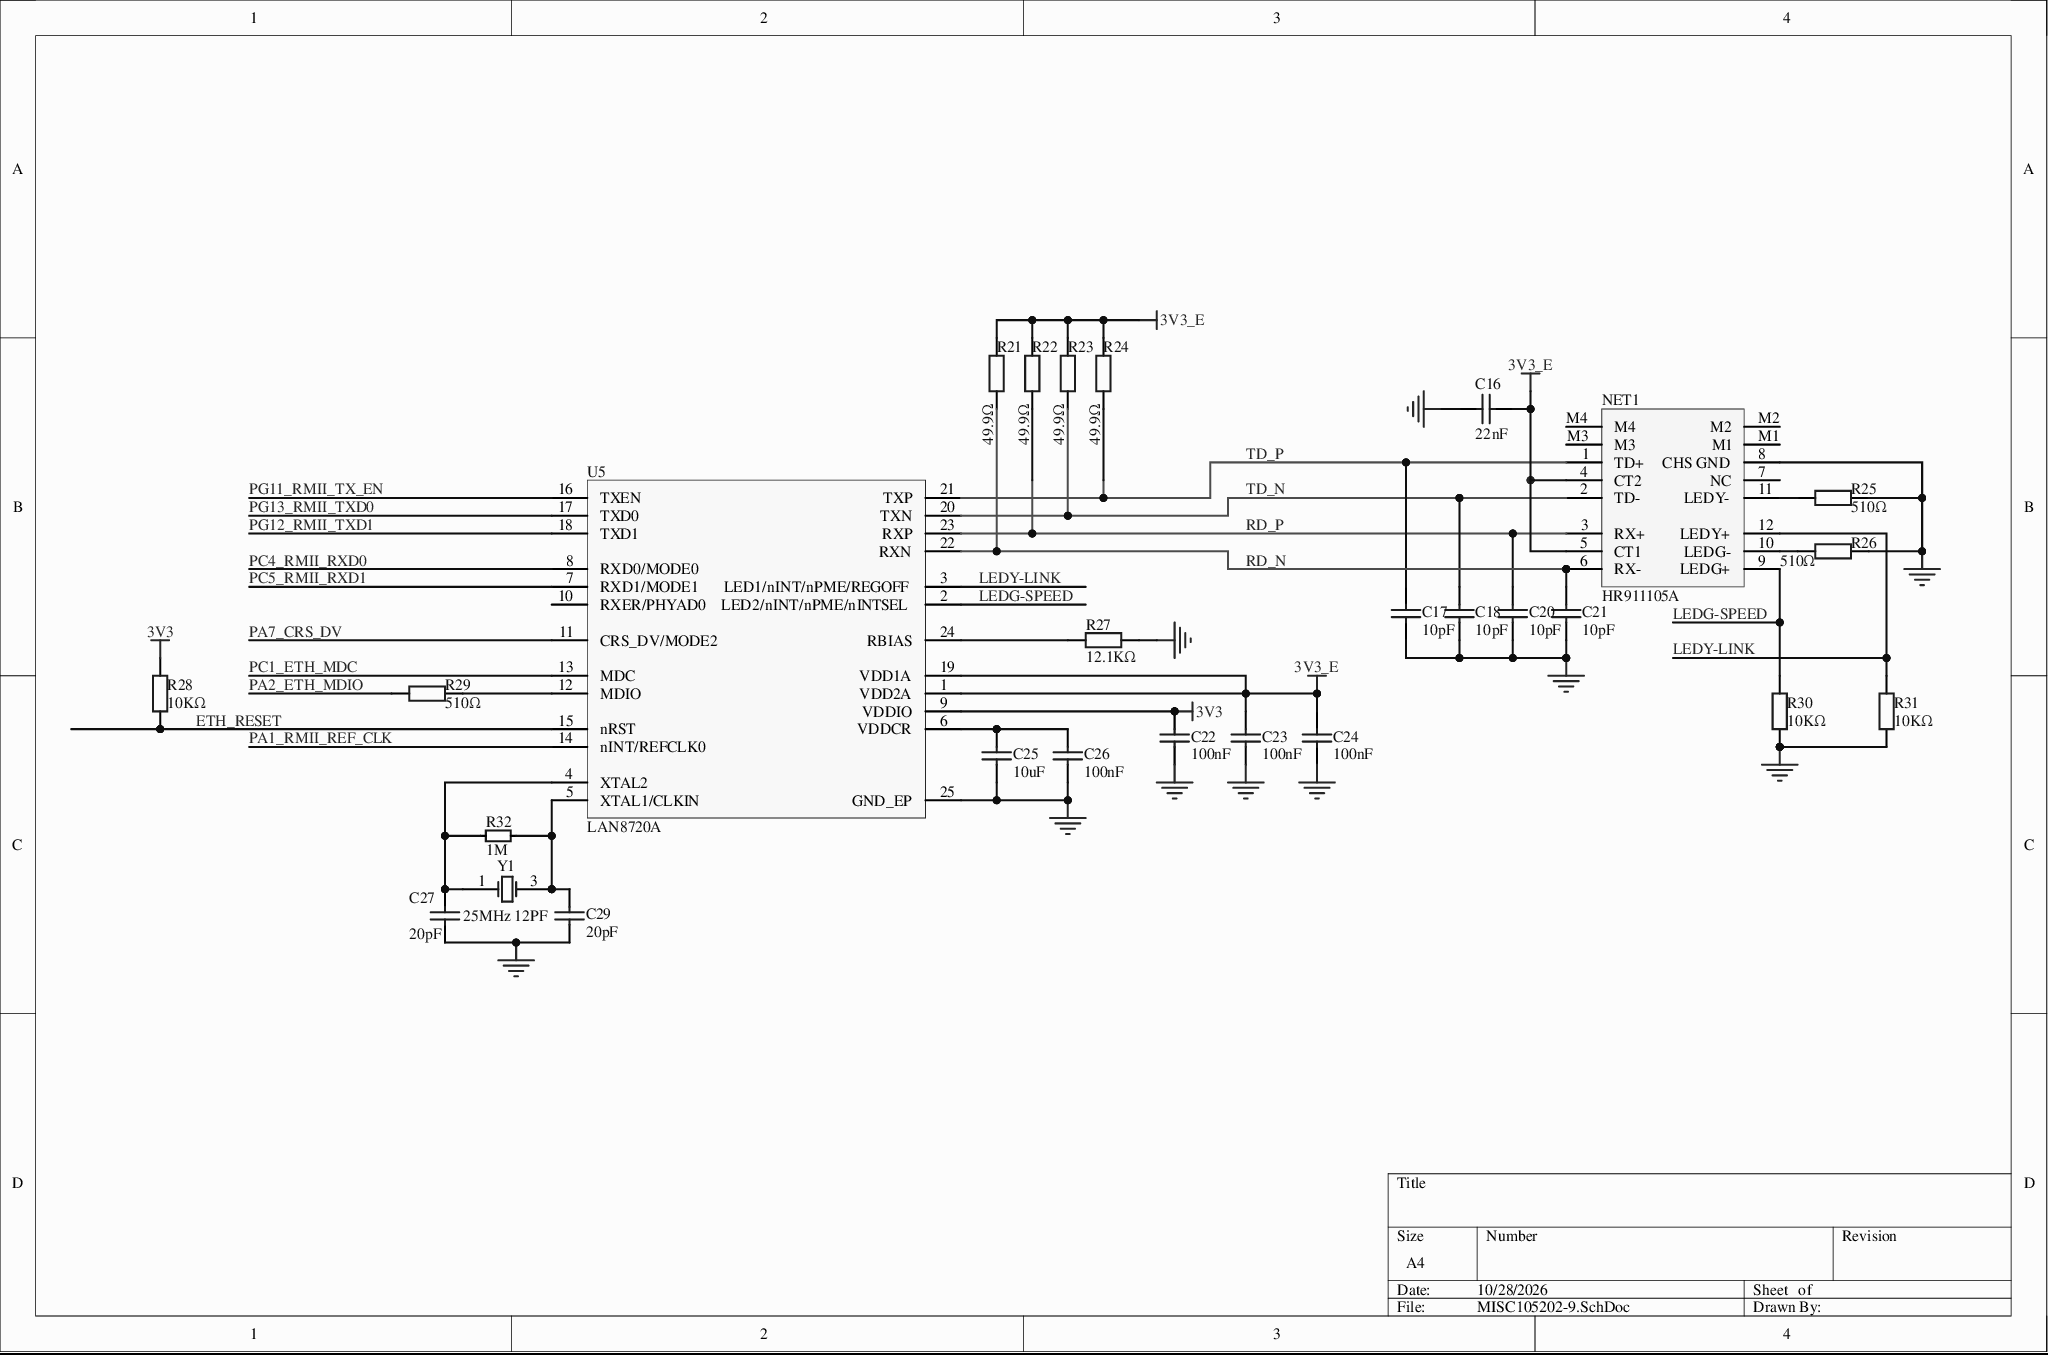
[diagram p0: MISC105202-9.SchDoc]
# Altium project MISC105202-19.PrjPCB (part 2 of 3)

## Sheet MISC105202-9.SchDoc
size A4

### Parts
C16  22nF  [0603_C]
C17  10pF  [0603_C]
C18  10pF  [0603_C]
C20  10pF  [0603_C]
C21  10pF  [0603_C]
C22  100nF  [0603_C]
C23  100nF  [0603_C]
C24  100nF  [0603_C]
C25  10uF  [0603_C]
C26  100nF  [0603_C]
C27  20pF  [0402_C]
C29  20pF  [0402_C]
NET1  HR911105A  [RJ45]
R21  49.9Ω  [0603_R]
R22  49.9Ω  [0603_R]
R23  49.9Ω  [0603_R]
R24  49.9Ω  [0603_R]
R25  510Ω  [0603_R]
R26  510Ω  [0603_R]
R27  12.1KΩ  [0603_R]
R28  10KΩ  [0603_R]
R29  510Ω  [0603_R]
R30  10KΩ  [0603_R]
R31  10KΩ  [0603_R]
R32  1M  [0402_R]
U5  LAN8720A  [QFN-24_4X4x05P]
Y1  25MHz 12PF  [SMD-3225_4P]

### Nets
3V3: C22.2 R28.1 U5.9(VDDIO)
3V3_E: C16.1 C23.2 C24.2 NET1.4(CT2) NET1.5(CT1) R21.2 R22.2 R23.2 R24.2 U5.1(VDD2A) U5.19(VDD1A)
GND: C16.2 C17.2 C18.2 C20.2 C21.2 C22.1 C23.1 C24.1 C25.1 C26.1 C27.2 C29.2 NET1.8(CHS_GND) R25.2 R26.2 R27.2 R30.2 R31.1 U5.25(GND_EP)
ETH_RESET: R28.2 U5.15(nRST)
LEDG-SPEED: NET1.9(LEDG+) R30.1 U5.2(LED2/nINT/nPME/nINTSEL)
LEDY-LINK: NET1.12(LEDY+) R31.2 U5.3(LED1/nINT/nPME/REGOFF)
PA1_RMII_REF_CLK: U5.14(nINT/REFCLK0)
PA2_ETH_MDIO: R29.1
PA7_CRS_DV: U5.11(CRS_DV/MODE2)
PC1_ETH_MDC: U5.13(MDC)
PC4_RMII_RXD0: U5.8(RXD0/MODE0)
PC5_RMII_RXD1: U5.7(RXD1/MODE1)
PG11_RMII_TX_EN: U5.16(TXEN)
PG12_RMII_TXD1: U5.18(TXD1)
PG13_RMII_TXD0: U5.17(TXD0)
RD_N: C21.1 NET1.6(RX-) R21.1 U5.22(RXN)
RD_P: C20.1 NET1.3(RX+) R22.1 U5.23(RXP)
TD_N: C18.1 NET1.2(TD-) R23.1 U5.20(TXN)
TD_P: C17.1 NET1.1(TD+) R24.1 U5.21(TXP)
NetC25_2: C25.2 C26.2 U5.6(VDDCR)
NetC27_1: C27.1 R32.2 U5.4(XTAL2) Y1.1(OSC1)
NetC29_1: C29.1 R32.1 U5.5(XTAL1/CLKIN) Y1.3(OSC2)
NetNET1_10: NET1.10(LEDG-) R26.1
NetNET1_11: NET1.11(LEDY-) R25.1
NetR27_1: R27.1 U5.24(RBIAS)
NetR29_2: R29.2 U5.12(MDIO)

Not connected (* = marked no-connect by the designer): NET1 7(NC) M1 M2 M3 M4; U5 10(RXER/PHYAD0)

### Layout directives
differential pair: RD_N, RD_P, TD_N, TD_P
rule Matched Net Lengths [Tolerance = 100mil]: RD_N, RD_P, TD_N, TD_P

### Library data of the parts
C16 = 0603 22nF (223) 10% 50V: 贴片电容; ComponentLink1Description: supplier link; Package: 0603; Supplier: LC; SuppliersPartNumber: C21122
C17 C18 C20 C21 = 0603 10pF (100) 5% 50V: 贴片电容; ComponentLink1Description: supplier link; Package: 0603; Supplier: LC; SuppliersPartNumber: C1634
C22-C24 C26 = 0603 100nF (104) 10% 50V: 贴片电容; ComponentLink1Description: supplier link; Package: 0603; Supplier: LC; SuppliersPartNumber: C14663
C25 = 0603 10uF (106) 10% 10V: 贴片电容; ComponentLink1Description: supplier link; Package: 0603; Supplier: LC; SuppliersPartNumber: C19702
C27 C29 = Cap Semi: Capacitor (Semiconductor SIM Model); Published: 8-Jun-2000; LatestRevisionDate: 29-May-2009; LatestRevisionNote: IPC-7351 Footprint Added.; PackageReference: C1206; PackageDescription: Chip Capacitor; Publisher: Altium Limited
R21-R24 = 0603 49.9Ω (49R9) 1%: 贴片电阻; ComponentLink1Description: supplier link; Package: 0603; Supplier: LC; SuppliersPartNumber: C23185
R25 R26 R29 = 0603 510Ω (5100) 1%: 贴片电阻; ComponentLink1Description: supplier link; Package: 0603; Supplier: LC; SuppliersPartNumber: C23193
R27 = 0603 12KΩ (1202) 1%: 贴片电阻; ComponentLink1Description: supplier link; Package: 0603; Supplier: LC; SuppliersPartNumber: C22790
R28 R30 R31 = 0603 10KΩ (1002) 1%: 贴片电阻; ComponentLink1Description: supplier link; Package: 0603; Supplier: LC; SuppliersPartNumber: C25804
R32 = Reszte: Resistor
U5 = LAN8742A-CZ-TR: LAN8742A-CZ-TR - Small Footprint RMII 10/100 Ethernet, Transceiver with HP Auto-MDIX and flexPWR Technology SQFN-24; Manuf_1: MICROCHIP; Order: LAN8742A-CZ-TR; Manuf_Part_1: LAN8742A-CZ-TR; Distrib: MICROCHIP
Y1 = SMD-3225_4P  25MHZ 12PF 10PPM: 贴片晶振; ComponentLink1Description: supplier link; Package: SMD-3225_4P; Supplier: LC; SuppliersPartNumber: C9006

## Sheet MISC105202-21.SchDoc
size B
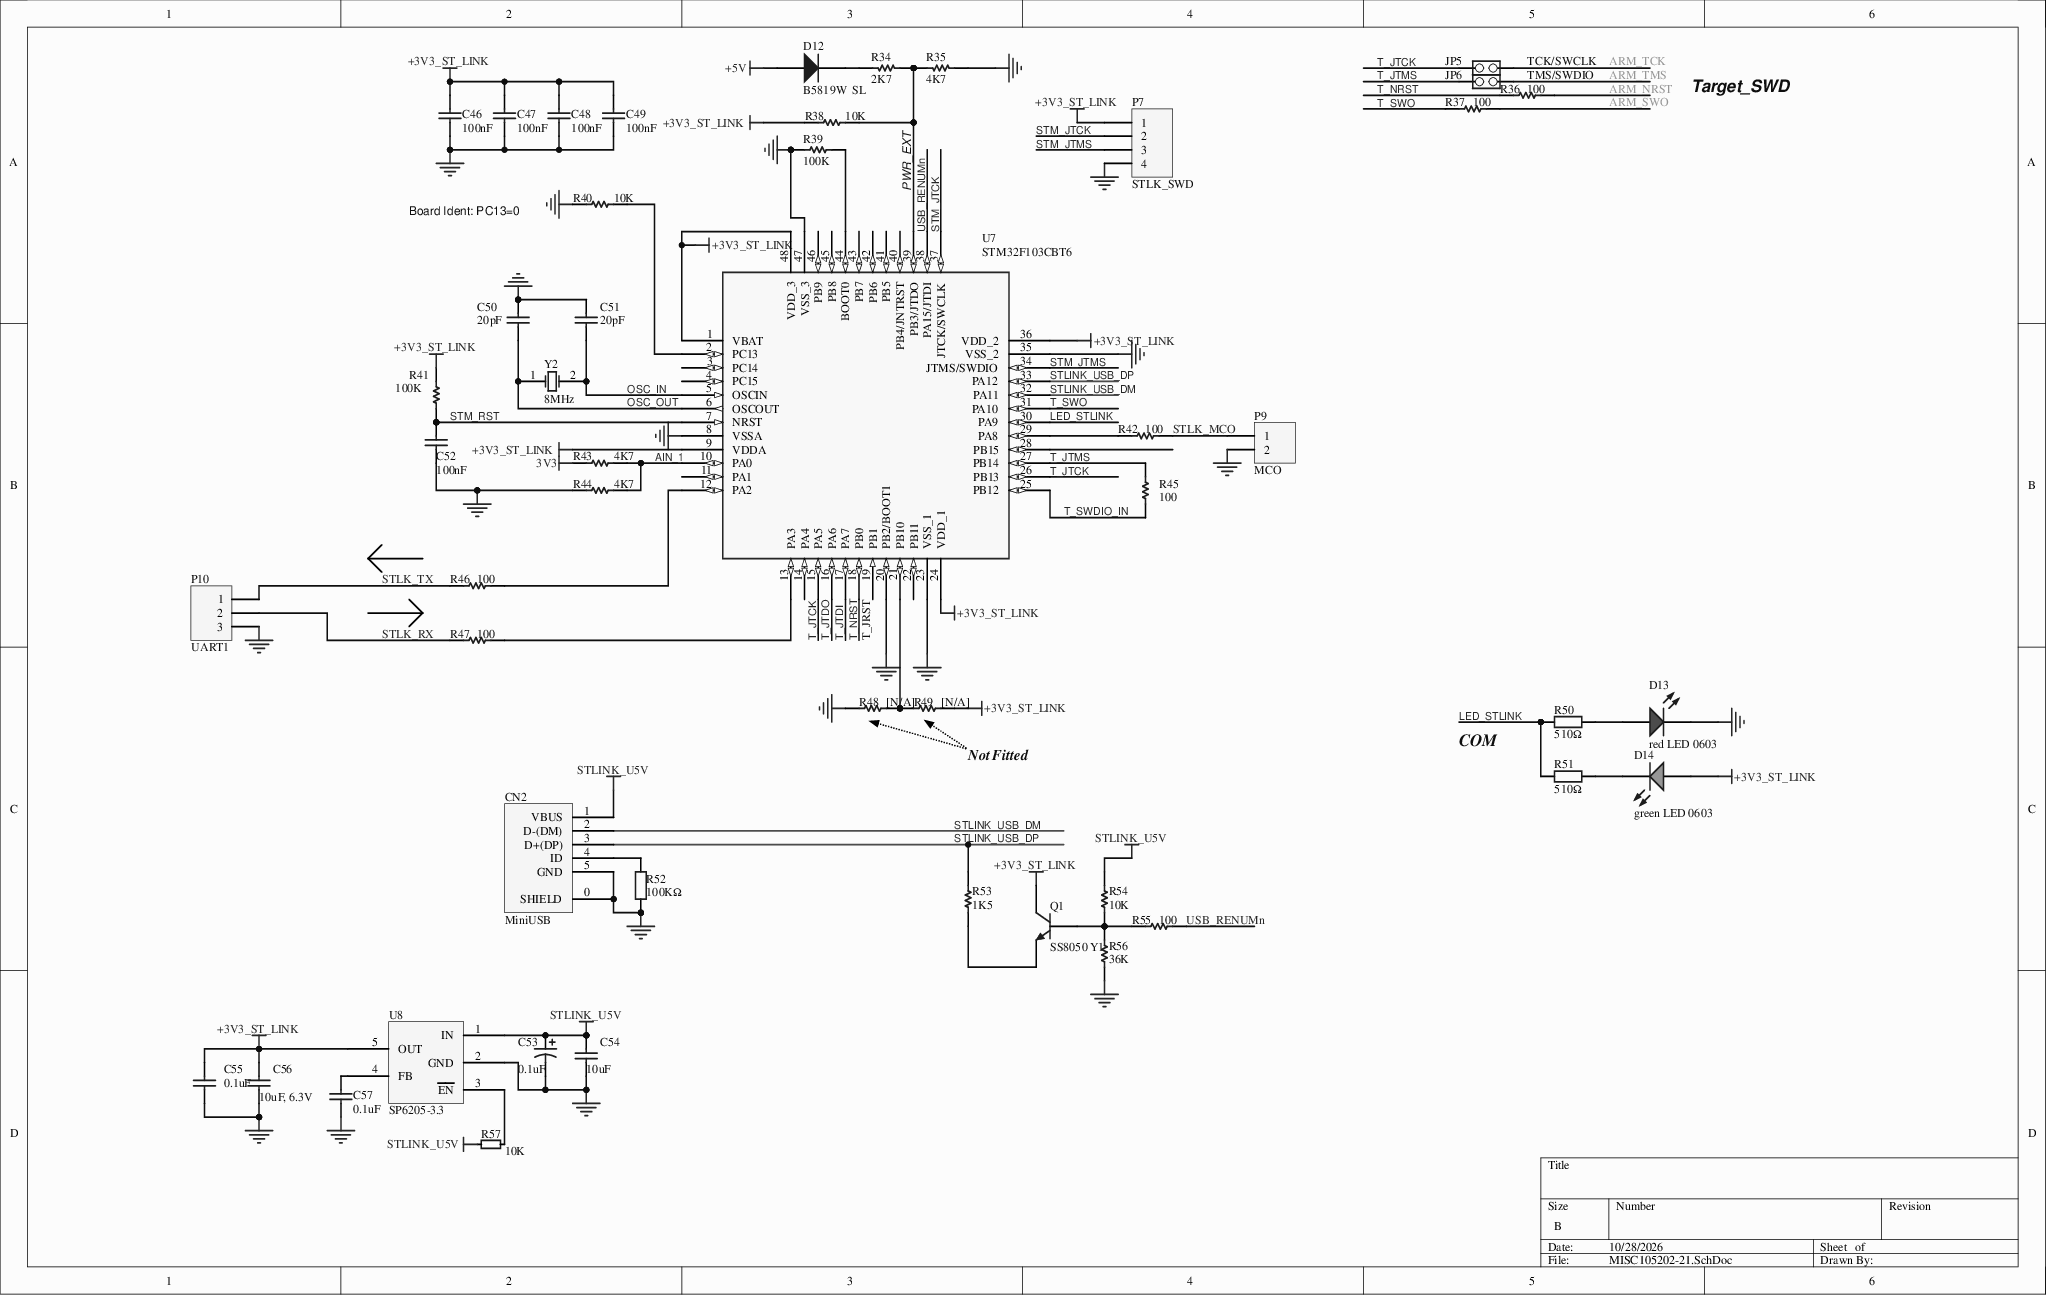
[diagram p1: MISC105202-21.SchDoc]

### Parts
C46  100nF  [0603_C]
C47  100nF  [0603_C]
C48  100nF  [0603_C]
C49  100nF  [0603_C]
C50  20pF  [0603_C]
C51  20pF  [0603_C]
C52  100nF  [0603_C]
C53  0.1uF  [0402_C]
C54  10uF  [0402_C]
C55  value 0.1uF  [0603_C]  (hidden comment: 0.1uF,25V)
C56  10uF, 6.3V  [0402_C]
C57  0.1uF  [0402_C]
CN2  MiniUSB  [Mini-USB-AB]
D12  B5819W  SL  [SOD-123]
D13  red LED 0603  [0603_LED_S1]
D14  green LED 0603  [0603_LED_S1]
JP5  (no value)  [HDR1X2]
JP6  (no value)  [HDR1X2]
P7  STLK_SWD  [127*4]
P9  MCO  [HDR1X2]
P10  UART1  [HDR1X3]
Q1  SS8050 Y1  [SOT-23(SOT-23-3)]
R34  2K7  [0603_R]
R35  4K7  [0603_R]
R36  100  [0603_R]
R37  100  [0603_R]
R38  10K  [0603_R]
R39  100K  [0603_R]
R40  10K  [0603_R]
R41  100K  [0603_R]
R42  100  [0603_R]
R43  4K7  [0603_R]
R44  4K7  [0603_R]
R45  100  [0603_R]
R46  100  [0603_R]
R47  100  [0603_R]
R48  [N/A]  [0603_R]
R49  [N/A]  [0603_R]
R50  510Ω  [0603_R]
R51  510Ω  [0603_R]
R52  100KΩ  [0603_R]
R53  1K5  [0603_R]
R54  10K  [0603_R]
R55  100  [0603_R]
R56  36K  [0603_R]
R57  10K  [0402_R]
U7  STM32F103CBT6  [LQFP-48_7x7x05P]
U8  SP6205-3.3  [SOT23-5]
Y2  8MHz  [SMD-5032_2P]

### Nets
3V3: R43.1
+3V3_ST_LINK: C46.2 C47.2 C48.2 C49.2 C55.2 C56.2 D14.A P7.1 Q1.3(C) R38.1 R41.2 R49.1 U7.1(VBAT) U7.9(VDDA) U7.24(VDD_1) U7.36(VDD_2) U7.48(VDD_3) U8.5(OUT)
+5V: D12.1(A)
GND: C46.1 C47.1 C48.1 C49.1 C50.2 C51.2 C52.1 C53.2 C54.1 C55.1 C56.1 C57.1 CN2.0(SHIELD) CN2.5(GND) D13.K P7.4 P9.2 P10.3 R35.2 R39.1 R40.1 R44.1 R48.2 R52.1 R56.1 U7.8(VSSA) U7.20(PB2/BOOT1) U7.23(VSS_1) U7.35(VSS_2) U7.47(VSS_3) U8.2(GND)
STLINK_U5V: C53.1 C54.2 CN2.1(VBUS) R54.2 R57.2 U8.1(IN)
AIN_1: R43.2 R44.2 U7.10(PA0)
ARM_NRST: R36.2
ARM_SWO: R37.2
ARM_TCK: JP5.2(NO)
ARM_TMS: JP6.2(NO)
LED_STLINK: R50.1 R51.1 U7.30(PA9)
OSC_IN: C51.1 U7.5(OSCIN) Y2.2(OSC2)
OSC_OUT: C50.1 U7.6(OSCOUT) Y2.1(OSC1)
STLINK_USB_DM: CN2.2(D-(DM)) U7.32(PA11)
STLINK_USB_DP: CN2.3(D+(DP)) R53.1 U7.33(PA12)
STLK_MCO: P9.1 R42.2
STLK_RX: P10.2 R47.1  [project net PA9_U1T]
STLK_TX: P10.1 R46.1  [project net PA10_U1R]
STM_JTCK: P7.2 U7.37(JTCK/SWCLK)
STM_JTMS: P7.3 U7.34(JTMS/SWDIO)
STM_RST: C52.2 R41.1 U7.7(NRST)
T_JTCK: JP5.1(COMMON) U7.15(PA5) U7.26(PB13)
T_JTDI: U7.17(PA7)
T_JTDO: U7.16(PA6)
T_JTMS: JP6.1(COMMON) R45.2 U7.27(PB14)
T_NRST: R36.1 U7.18(PB0)
T_SWDIO_IN: R45.1 U7.25(PB12)
T_SWO: R37.1 U7.31(PA10)
USB_RENUMn: R55.2 U7.38(PA15/JTDI)
NetC57_2: C57.2 U8.4(FB)
NetCN2_4: CN2.4(ID) R52.2
NetD12_2: D12.2(K) R34.1
NetD13_A: D13.A R50.2
NetD14_K: D14.K R51.2
NetQ1_1: Q1.1(B) R54.1 R55.1 R56.2
NetQ1_2: Q1.2(E) R53.2
NetR34_2: R34.2 R35.1 R38.2 U7.39(PB3/JTDO)
NetR39_2: R39.2 U7.44(BOOT0)
NetR40_2: R40.2 U7.2(PC13)
NetR42_1: R42.1 U7.29(PA8)
NetR46_2: R46.2 U7.12(PA2)
NetR47_2: R47.2 U7.13(PA3)
NetR48_1: R48.1 R49.2 U7.21(PB10)
NetR57_1: R57.1 U8.3(~{EN})

Not connected (* = marked no-connect by the designer): U7 3(PC14) 4(PC15)* 11(PA1)* 14(PA4)* 19(PB1)* 22(PB11)* 28(PB15) 40(PB4/JNTRST)* 41(PB5)* 42(PB6)* 43(PB7)* 45(PB8)* 46(PB9)*

### Layout directives
differential pair: (no net found under the mark)
mark named Diff Pair 90ohm: STLINK_USB_DM, STLINK_USB_DP

### Notes on the sheet
- TCK/SWCLK
- (near R36) TMS/SWDIO
- Target_SWD
- Board Ident: PC13=0
- PWR_EXT
- T_JRST
- (near R49) Not Fitted
- COM

### Library data of the parts
C46-C49 C52 = Capacitor_ST: Capacitor 0402 / 0603 / 0805; Revision: July-2002: Re-released for DXP Platform.; Value: 100nF
C50 C51 = Capacitor_ST: Capacitor 0402 / 0603 / 0805; Value: 100nF; Revision: July-2002: Re-released for DXP Platform.
C53 = Cap Pol1: Polarized Capacitor (Radial); Published: 8-Jun-2000; LatestRevisionDate: 17-Jul-2002; LatestRevisionNote: Re-released for DXP Platform.; PackageReference: RB7.6-15; Publisher: Altium Limited
C54 C55 C57 = Cap Semi: Capacitor (Semiconductor SIM Model); Published: 8-Jun-2000; LatestRevisionDate: 29-May-2009; LatestRevisionNote: IPC-7351 Footprint Added.; PackageReference: C1206; PackageDescription: Chip Capacitor; Publisher: Altium Limited
C56 = 0402 10uF (106) 20% 6.3V: 贴片电容; ComponentLink1Description: supplier link; Package: 0402; Supplier: LC; SuppliersPartNumber: C15525
CN2 = Mini-USB-AB
D12 = SOD-123 B5819W  SL: 肖特基二极管; ComponentLink1Description: supplier link; Package: SOD-123; Supplier: LC; SuppliersPartNumber: C8598
D13 = 0603 红灯: 发光二极管; ComponentLink1Description: supplier link; Package: 0603; Supplier: LC; SuppliersPartNumber: C2286
D14 = 0603 绿灯: 发光二极管; ComponentLink1Description: supplier link; Package: 0603; Supplier: LC; SuppliersPartNumber: C72043
JP5 JP6 = JP2
P7 = Header 4: Header, 4-Pin; LatestRevisionDate: 17-Jul-2002; LatestRevisionNote: Re-released for DXP Platform.; Publisher: Altium Limited
P9 = Header 2: Header, 2-Pin; LatestRevisionDate: 17-Jul-2002; LatestRevisionNote: Re-released for DXP Platform.; Publisher: Altium Limited
P10 = Header 3: Header, 3-Pin; LatestRevisionDate: 17-Jul-2002; LatestRevisionNote: Re-released for DXP Platform.; Publisher: Altium Limited
Q1 = SOT-23 SS8050 Y1: 三极管; ComponentLink1Description: supplier link; Package: SOT-23; Supplier: LC; SuppliersPartNumber: C2150
R34 R35 R48 R49 R54 R56 = Res1: Resistor; Value: 1K; Published: 8-Jun-2000; Revision: July-2002: Re-released for DXP Platform.; Publisher: Altium Limited
R36 R37 R39 R41 R42 R45-R47 R53 R55 = Resistor_ST: Resistor 0402 / 0603 / 0805; Value: 10K
R38 R40 = Resistor_ST: Resistor 0402 / 0603 / 0805; Value: 10K
R43 R44 = Resistor_ST: Resistor 0402 / 0603 / 0805; Value: 10K; Fitted: NO
R50 R51 = 0603 510Ω (5100) 1%: 贴片电阻; ComponentLink1Description: supplier link; Package: 0603; Supplier: LC; SuppliersPartNumber: C23193
R52 = 0603 10KΩ (1002) 1%: 贴片电阻; ComponentLink1Description: supplier link; Package: 0603; Supplier: LC; SuppliersPartNumber: C25804
R57 = Reszte: Resistor
U7 = STM32F103CBT6: Medium-density performance line ARM-based 32-bit MCU with 64KB Flash; Manuf_Part_1: STM32F103C8T6; Manuf_1: STM; Ref St: 9175981; Provided: ST; ECCN_US/EU: 3A991A2/NEC; Footprint: QFP48 7X7; Distrib: ST; Order: STM32F103C8T6
U8 = TPS76901HDB
Y2 = SMD-5032_2P 8MHz 20ppm 20pF: 贴片晶振; ComponentLink1Description: supplier link; Package: SMD-5032_2P; Supplier: LC; SuppliersPartNumber: C115962

## Sheet MISC105202-13.SchDoc
size A4
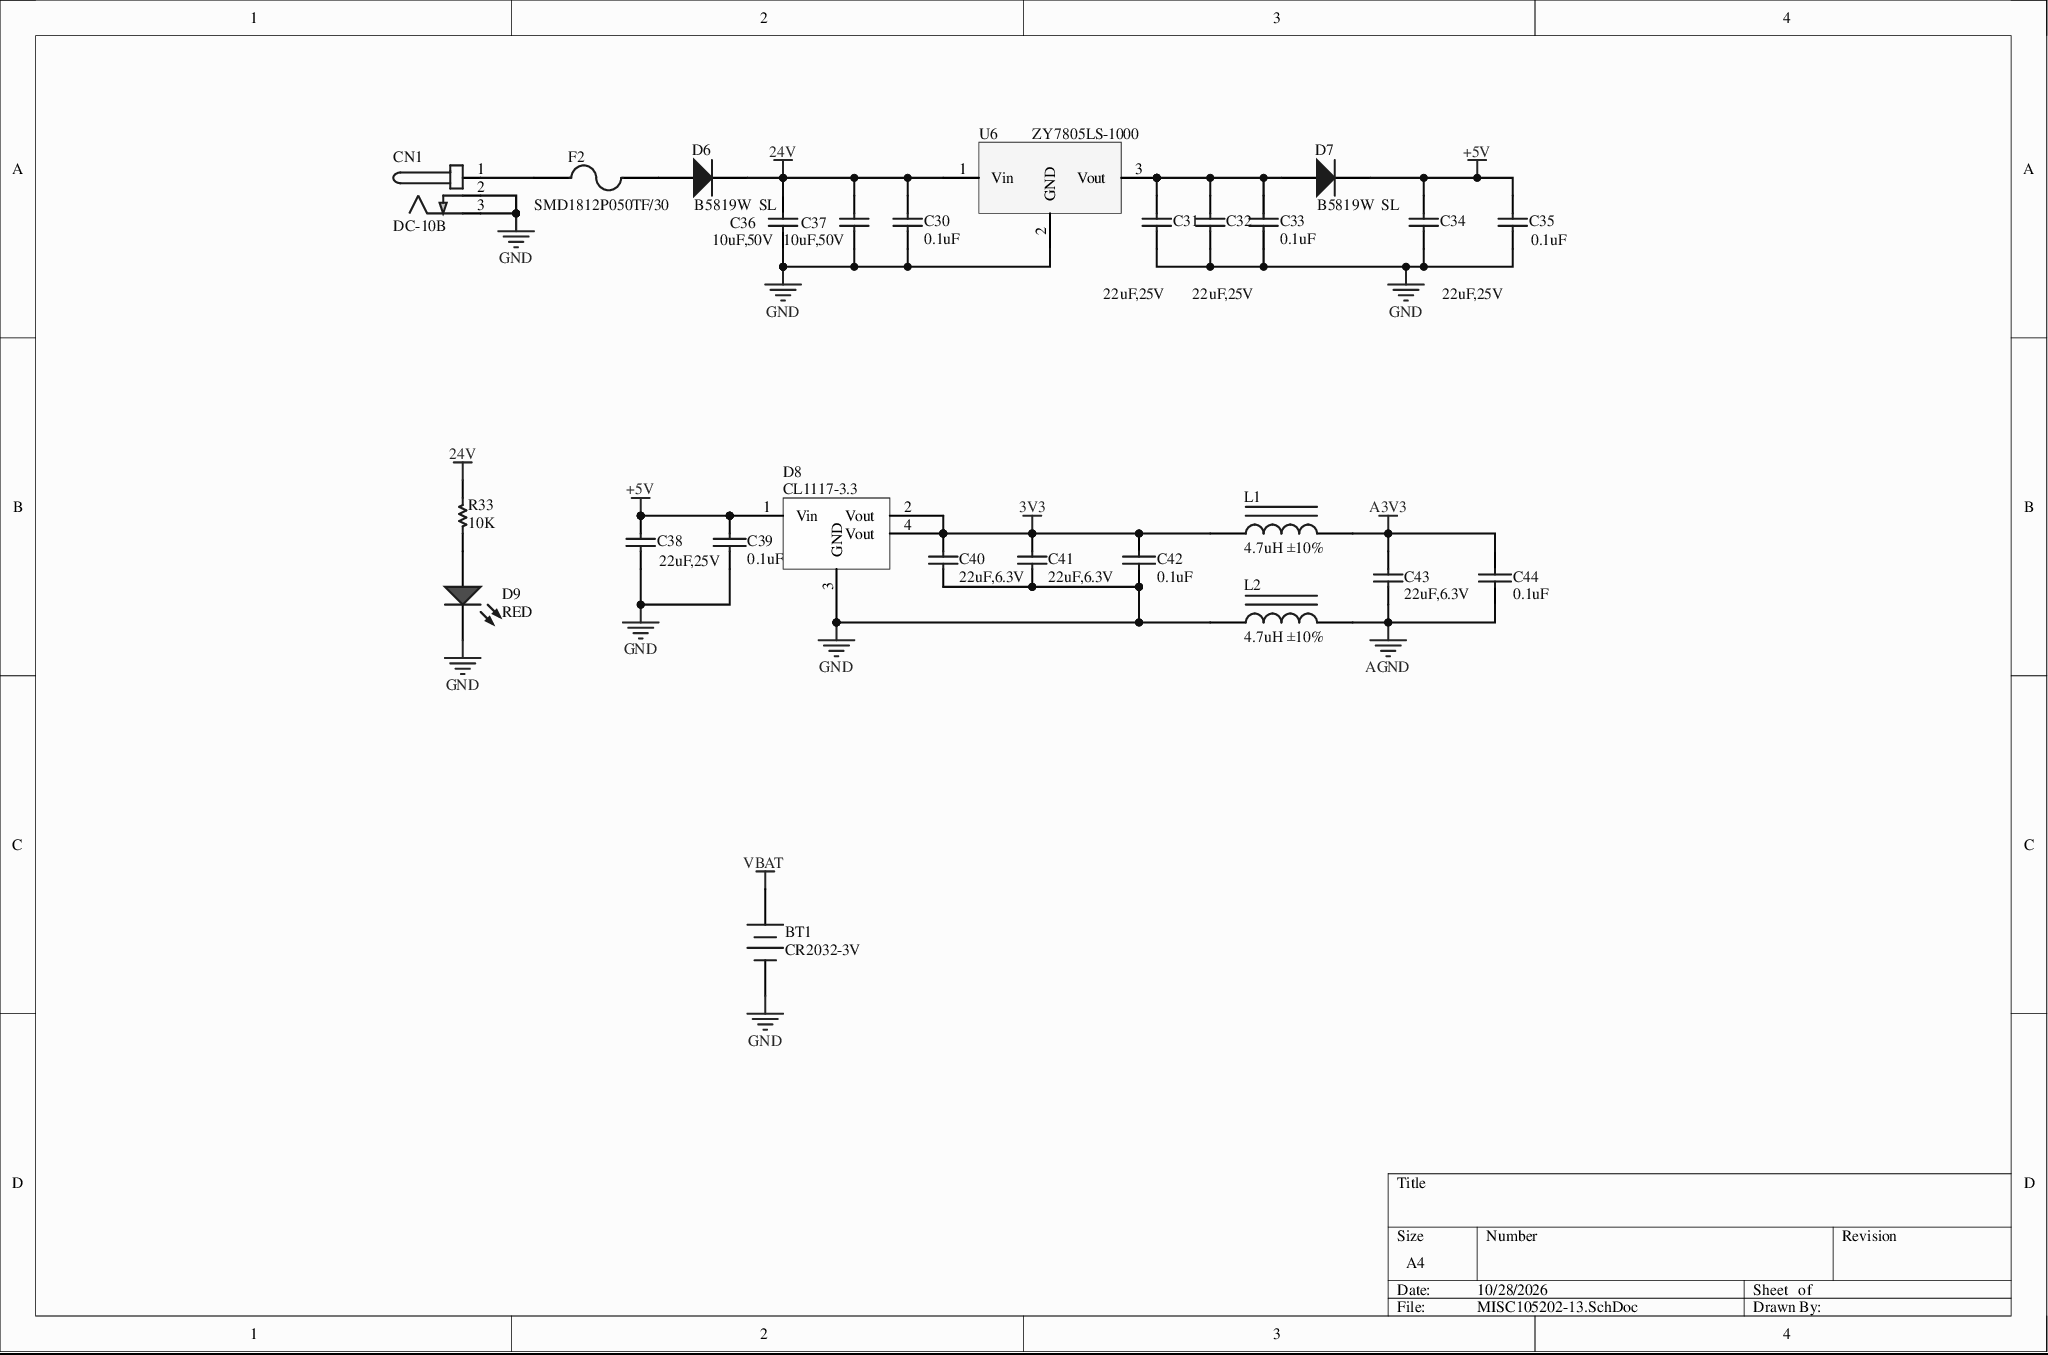
[diagram p2: MISC105202-13.SchDoc]

### Parts
BT1  CR2032-3V  [BT1]
C30  0.1uF  [0402_C]
C31  22uF,25V  [0805_C]
C32  22uF,25V  [0805_C]
C33  0.1uF  [0402_C]
C34  22uF,25V  [0805_C]
C35  0.1uF  [0402_C]
C36  10uF,50V  [1206_C]
C37  10uF,50V  [1206_C]
C38  22uF,25V  [0805_C]
C39  0.1uF  [0603]
C40  22uF,6.3V  [0603_C]
C41  22uF,6.3V  [0603_C]
C42  0.1uF  [0603]
C43  22uF,6.3V  [0603_C]
C44  0.1uF  [0603]
CN1  DC-10B  [DC10B]
D6  B5819W  SL  [SOD-123]
D7  B5819W  SL  [SOD-123]
D8  CL1117-3.3  [SOT-223]
D9  RED  [0603_LED_S1]
F2  SMD1812P050TF/30  [1812]
L1  4.7uH ±10%  [0603_L]
L2  4.7uH ±10%  [0603_L]
R33  10K  [0603]
U6  ZY7805LS-1000  [ZY78xxLS-1000]

### Nets
3V3: C40.2 C41.2 C42.2 D8.2(Vout) D8.4(Vout) L1.1
24V: C30.1 C36.2 C37.2 D6.2(K) R33.1 U6.1(Vin)  [project net AIN2]
+5V: C34.2 C35.1 C38.2 C39.2 D7.2(K) D8.1(Vin)
A3V3: C43.2 C44.2 L1.2
AGND: C43.1 C44.1 L2.2
GND: BT1.2(-) C30.2 C31.1 C32.1 C33.2 C34.1 C35.2 C36.1 C37.1 C38.1 C39.1 C40.1 C41.1 C42.1 CN1.2(GND) CN1.3(GND) D8.3(GND) D9.K L2.1 U6.2(GND)
VBAT: BT1.1(+)
NetC31_2: C31.2 C32.2 C33.1 D7.1(A) U6.3(Vout)
NetCN1_1: CN1.1(+) F2.2
NetD6_1: D6.1(A) F2.1
NetD9_A: D9.A R33.2

### Library data of the parts
BT1 = Battery: Multicell Battery; Published: 24-Mar-1999; LatestRevisionDate: 17-Jul-2002; LatestRevisionNote: Re-released for DXP Platform.; PackageReference: BAT-2; PackageDescription: Battery; 2 Leads; Publisher: Altium Limited
C30 C33 C35 = 0402 100nF (104) 10% 16V: 贴片电容; ComponentLink1Description: supplier link; Package: 0402; Supplier: LC; SuppliersPartNumber: C1525
C31 C32 C34 C38 = 0805 22uF (226) 20% 25V: 贴片电容; ComponentLink1Description: supplier link; Package: 0805; Supplier: LC; SuppliersPartNumber: C45783
C36 C37 = 1206 10uF (106) 10% 50V: 贴片电容; ComponentLink1Description: supplier link; Package: 1206; Supplier: LC; SuppliersPartNumber: C13585
C39 C42 C44 = CAP: Capacitor
C40 C41 C43 = 0603 22uF (226) 20% 6.3V: 贴片电容; ComponentLink1Description: supplier link; Package: 0603; Supplier: LC; SuppliersPartNumber: C59461
CN1 = PJ202A
D6 D7 = SOD-123 B5819W  SL: 肖特基二极管; ComponentLink1Description: supplier link; Package: SOD-123; Supplier: LC; SuppliersPartNumber: C8598
D8 = CL1117-33
D9 = 0603 红灯: 发光二极管; ComponentLink1Description: supplier link; Package: 0603; Supplier: LC; SuppliersPartNumber: C2286
F2 = Fuse 2: Fuse; Published: 8-Jun-2000; LatestRevisionDate: 17-Jul-2002; LatestRevisionNote: Re-released for DXP Platform.; PackageReference: PIN-W2/E2.8; Publisher: Altium Limited
L1 L2 = 0603 4.7uH 10%: 贴片电感; ComponentLink1Description: supplier link; Package: 0603; Supplier: LC; SuppliersPartNumber: C1034
R33 = RES-S
U6 = ZY78xxLS